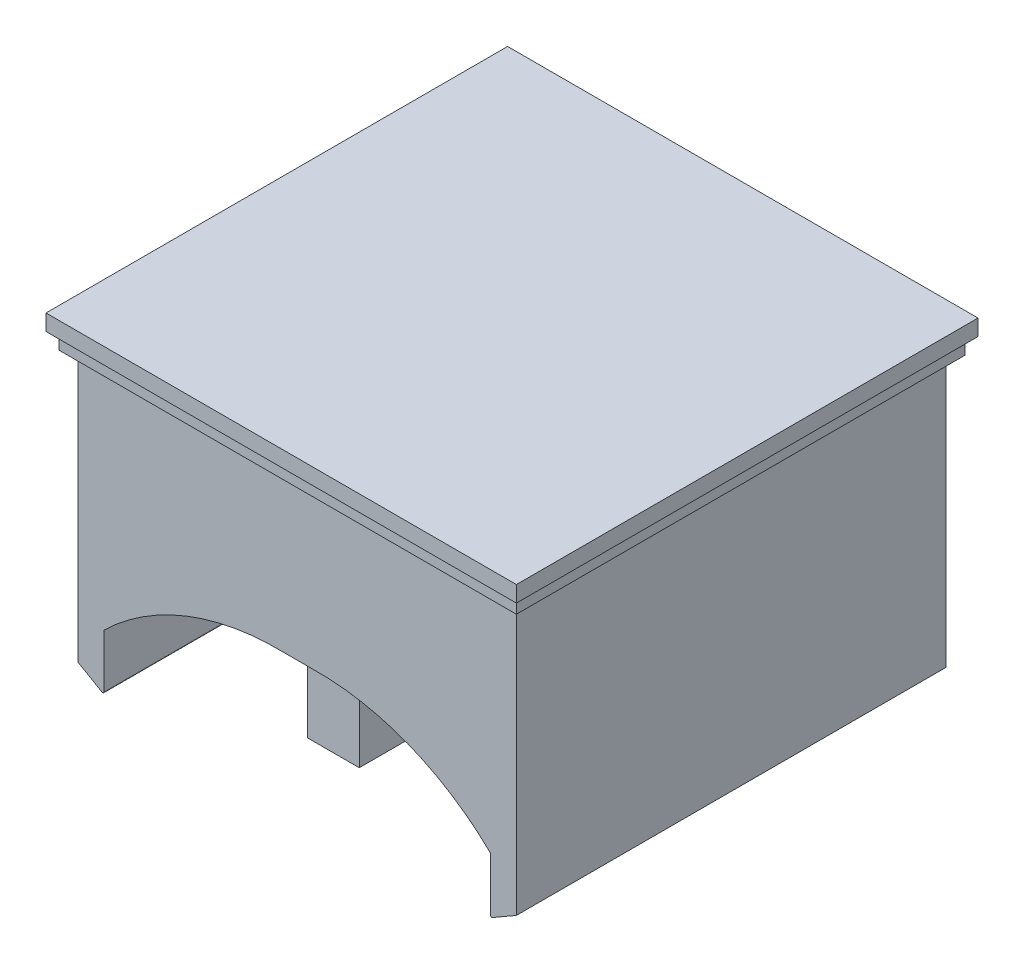
from build123d import *

# Parameters (mm, degrees)
BOSS_EXTRUDE1_DEPTH = 66.78
SKETCH3_W           = 8.06
SKETCH3_H           = 55.56
BOSS_EXTRUDE2_DEPTH = 40
SKETCH5_W           = 71.144376366
SKETCH5_H           = 69.78
BOSS_EXTRUDE4_DEPTH = 2.5
SKETCH6_W           = 73.144376366
SKETCH6_H           = 71.78
BOSS_EXTRUDE5_DEPTH = 2.5
SKETCH7_R           = 1.5
CUT_EXTRUDE1_DEPTH  = 10


with BuildPart() as part:
    # Sketch1 → Boss-Extrude1 (new body)
    with BuildSketch(Plane.XY):
        with BuildLine():
            Line((-34.072188183, 25.498094011), (34.072188183, 25.498094011))
            Line((34.072188183, 25.498094011), (34.072188183, -16.561905989))
            Line((34.072188183, -16.561905989), (30.370310886, -18.699185843))
            ThreePointArc((30.370310886, -18.699185843), (30.140310886, -18.699185843), (30.025310886, -18.5))
            Line((30.025310886, -18.5), (30.025310886, -10.173149416))
            ThreePointArc((30.025310886, -10.173149416), (17.215197166, -1.899763481), (2.201193992, 0.77))
            Line((2.201193992, 0.77), (0, 0.77))
            Line((0, 0.77), (-2.201193992, 0.77))
            ThreePointArc((-2.201193992, 0.77), (-17.215197166, -1.899763481), (-30.025310886, -10.173149416))
            Line((-30.025310886, -10.173149416), (-30.025310886, -18.5))
            ThreePointArc((-30.025310886, -18.5), (-30.140310886, -18.699185843), (-30.370310886, -18.699185843))
            Line((-30.370310886, -18.699185843), (-34.072188183, -16.561905989))
            Line((-34.072188183, -16.561905989), (-34.072188183, 25.498094011))
        make_face()
    extrude(amount=-BOSS_EXTRUDE1_DEPTH)

    # Sketch3 → Boss-Extrude2 (add)
    with BuildSketch(Plane(origin=(0, 25.498094011, 0), x_dir=(1, 0, 0), z_dir=(0, 1, 0))):
        with Locations((0, 33.39)):
            Rectangle(SKETCH3_W, SKETCH3_H)
    extrude(amount=-BOSS_EXTRUDE2_DEPTH)

    # Sketch5 → Boss-Extrude4 (add)
    with BuildSketch(Plane(origin=(0, 25.498094011, 0), x_dir=(1, 0, 0), z_dir=(0, 1, 0))):
        with Locations((0, 33.39)):
            Rectangle(SKETCH5_W, SKETCH5_H)
    extrude(amount=BOSS_EXTRUDE4_DEPTH)

    # Sketch6 → Boss-Extrude5 (add)
    with BuildSketch(Plane(origin=(0, 27.998094011, 0), x_dir=(1, 0, 0), z_dir=(0, 1, 0))):
        with Locations((0, 33.39)):
            Rectangle(SKETCH6_W, SKETCH6_H)
    extrude(amount=BOSS_EXTRUDE5_DEPTH)

    # Sketch7 → Cut-Extrude1 (cut)
    with BuildSketch(Plane(origin=(0, 0, -66.78), x_dir=(-1, 0, 0), z_dir=(0, 0, -1))):
        with Locations((0, 6.101165809)):
            Circle(SKETCH7_R)
        with Locations((0, 16.101165809)):
            Circle(SKETCH7_R)
    extrude(amount=-CUT_EXTRUDE1_DEPTH, mode=Mode.SUBTRACT)


solid = part.part
